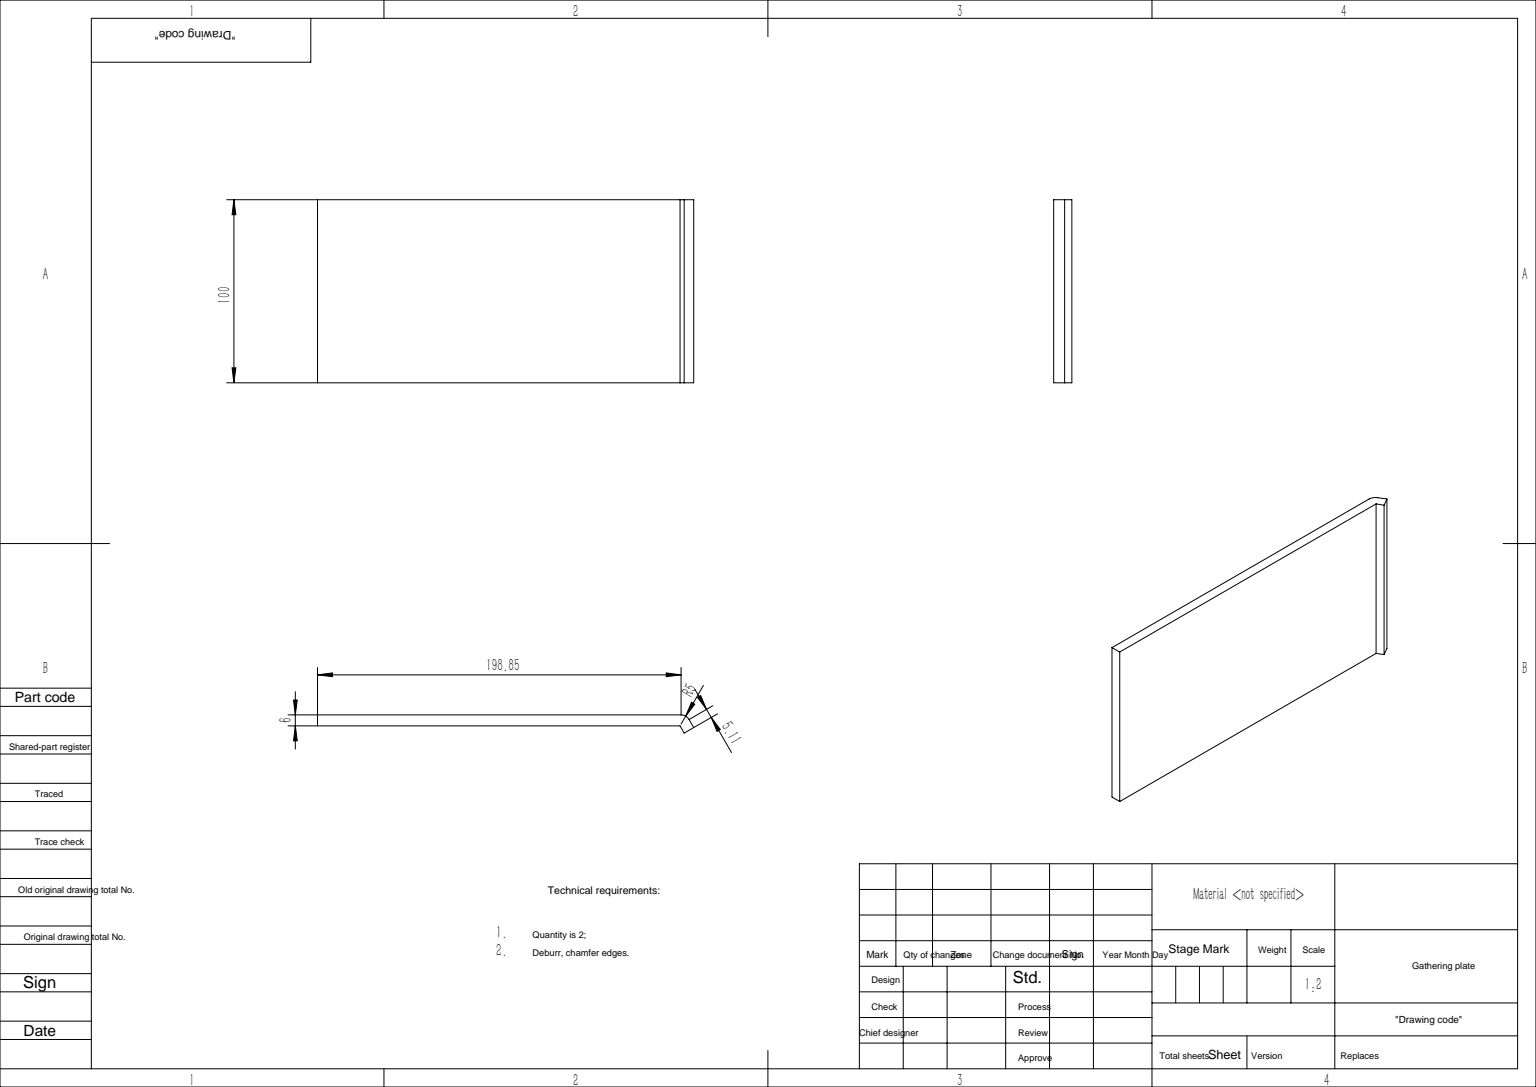
from build123d import *

# Parameters (mm, degrees)
EXTRUDE_1_DEPTH = 100
FILLET_1_R      = 5


with BuildPart() as part:
    # 草图1 → 凸台-拉伸1 (new body)
    with BuildSketch(Plane(origin=(0, 0, 0), x_dir=(1, 0, 0), z_dir=(0, 1, 0))):
        Polygon((3, 0), (3, 198.267949192), (6.92820323, 200.535898385), (3.92820323, 205.732050808), (-3, 201.732050808), (-3, 0), align=None)
    extrude(amount=EXTRUDE_1_DEPTH)

    # 圆角1
    fillet_1_edges = [part.edges().sort_by_distance(p)[0] for p in [
        (-3, 50, -201.732050808),
    ]]
    fillet(fillet_1_edges, radius=FILLET_1_R)


solid = part.part
